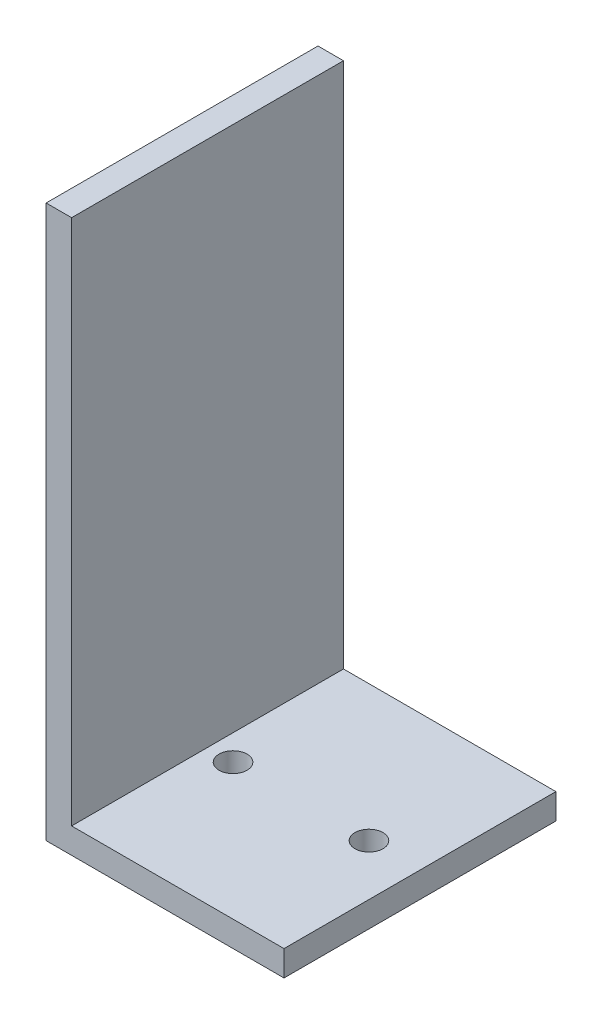
SolidWorks part; units mm, degrees
ref_plane "前视基准面" through (0, 0, 0) normal (0, 0, 1) x (1, 0, 0)
ref_plane "上视基准面" through (0, 0, 0) normal (0, 1, 0) x (1, 0, 0)
ref_plane "右视基准面" through (0, 0, 0) normal (1, 0, 0) x (0, 0, -1)
other "Configuration Table"
sketch "草图1" plane through (0, 0, 0) normal (0, 0, 1) x (1, 0, 0)
  line L0 (0, 0) -> (28, 0)
  line L1 (28, 0) -> (28, 3)
  line L2 (28, 3) -> (3, 3)
  line L3 (3, 3) -> (3, 65)
  line L4 (3, 65) -> (0, 65)
  line L5 (0, 65) -> (0, 0)
  point P0 (0, 0)
  dimension "D1" = 25
  dimension "D2" = 28
  dimension "D3" = 62
  dimension "D4" = 65
extrude "凸台-拉伸1" add sketch "草图1" against normal mid plane 32
sketch "草图2" plane through (0, 0, 0) normal (0, 1, 0) x (1, 0, 0)
  circle A0 centre (6, 0) radius 1.65
  circle A1 centre (22, 0) radius 1.65
  point P0 (0, 0)
  dimension "D1" = 3.3
  dimension "D2" = 3.3
  dimension "D3" = 6
  dimension "D4" = 22
extrude "切除-拉伸1" cut sketch "草图2" against normal mid plane 15
